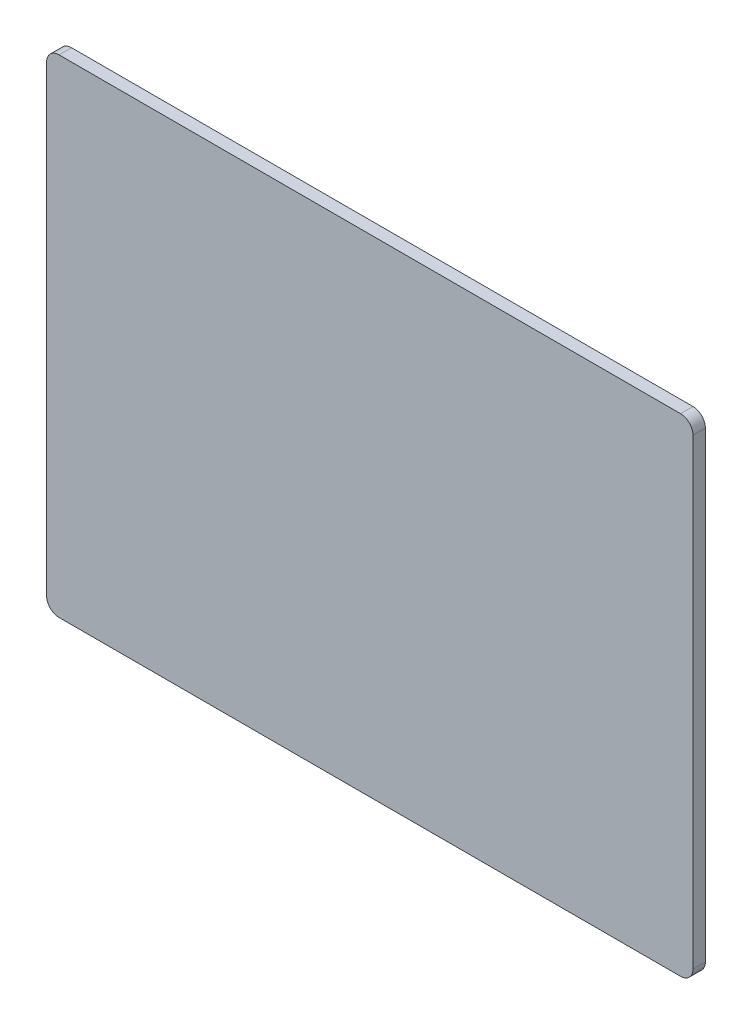
from build123d import *

# Parameters (mm, degrees)
SKETCH1_W           = 260
SKETCH1_H           = 196
BOSS_EXTRUDE1_DEPTH = 5
FILLET1_R           = 5


with BuildPart() as part:
    # Sketch1 → Boss-Extrude1 (new body)
    with BuildSketch(Plane.XY):
        with Locations((130, -98)):
            Rectangle(SKETCH1_W, SKETCH1_H)
    extrude(amount=BOSS_EXTRUDE1_DEPTH)

    # Fillet1
    fillet1_edges = [part.edges().sort_by_distance(p)[0] for p in [
        (0, 0, 2.5),
        (260, 0, 2.5),
        (260, -196, 2.5),
        (0, -196, 2.5),
    ]]
    fillet(fillet1_edges, radius=FILLET1_R)


solid = part.part
